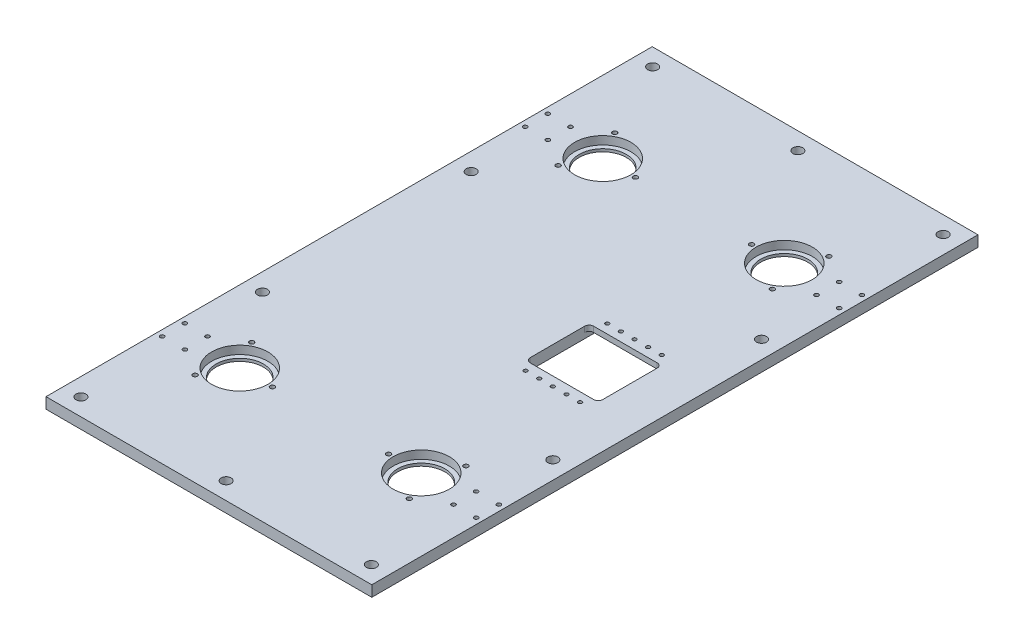
from build123d import *

# Parameters (mm, degrees)
SKETCH1_W                                          = 359
SKETCH1_H                                          = 668
BOSS_EXTRUDE1_DEPTH                                = 12
HOLE_SIZE_BASED_ON_SOCKET_HEAD_CAP_SCR_D           = 4.5
HOLE_SIZE_BASED_ON_SOCKET_HEAD_CAP_SCR_CBORE_D     = 8
HOLE_SIZE_BASED_ON_SOCKET_HEAD_CAP_SCR_CBORE_DEPTH = 4.6
SKETCH5_R                                          = 31
CUT_EXTRUDE2_DEPTH                                 = 9
SKETCH7_R                                          = 26
CUT_EXTRUDE4_DEPTH                                 = 380.368224816
M6_TAPPED_HOLE1_D                                  = 5
M6_TAPPED_HOLE1_DEPTH                              = 15
M6_TAPPED_HOLE1_TIP                                = 1.502151548
SKETCH12_R                                         = 5.5
CUT_EXTRUDE5_DEPTH                                 = 380.368224816
CUT_EXTRUDE6_DEPTH                                 = 380.368224816
CUT_EXTRUDE8_DEPTH                                 = 6
M5_TAPPED_HOLE1_D                                  = 4.2
M5_TAPPED_HOLE1_DEPTH                              = 12.4
M5_TAPPED_HOLE1_TIP                                = 1.2618073


with BuildPart() as part:
    # Sketch1 → Boss-Extrude1 (new body)
    with BuildSketch(Plane(origin=(0, 0, 0), x_dir=(1, 0, 0), z_dir=(0, 1, 0))):
        Rectangle(SKETCH1_W, SKETCH1_H)
    extrude(amount=BOSS_EXTRUDE1_DEPTH)

    # Hole size (%based on) socket head cap screw type 1 (through all)
    with Locations(Plane.XZ):
        with Locations((-173, 212.5), (-148, 212.5), (-148, 187.5), (-173, 187.5), (-173, -187.5), (-148, -187.5), (-148, -212.5), (-173, -212.5), (173, -212.5), (148, -212.5), (148, -187.5), (173, -187.5), (173, 187.5), (148, 187.5), (148, 212.5), (173, 212.5)):
            CounterBoreHole(HOLE_SIZE_BASED_ON_SOCKET_HEAD_CAP_SCR_D / 2, HOLE_SIZE_BASED_ON_SOCKET_HEAD_CAP_SCR_CBORE_D / 2, HOLE_SIZE_BASED_ON_SOCKET_HEAD_CAP_SCR_CBORE_DEPTH)

    # Sketch5 → Cut-Extrude2 (cut)
    with BuildSketch(Plane(origin=(0, 12, 0), x_dir=(1, 0, 0), z_dir=(0, 1, 0))):
        with Locations(Location((-100, -200, 0), (0, 0, 270))):
            Circle(SKETCH5_R)
        with Locations(Location((100, -200, 0), (0, 0, 90))):
            Circle(SKETCH5_R)
        with Locations(Location((100, 200, 0), (0, 0, 270))):
            Circle(SKETCH5_R)
        with Locations(Location((-100, 200, 0), (0, 0, 90))):
            Circle(SKETCH5_R)
    extrude(amount=-CUT_EXTRUDE2_DEPTH, mode=Mode.SUBTRACT)

    # Sketch7 → Cut-Extrude4 (cut, through all)
    with BuildSketch(Plane(origin=(0, 12, 0), x_dir=(1, 0, 0), z_dir=(0, 1, 0))):
        with Locations(Location((-100, 200, 0), (0, 0, 270))):
            Circle(SKETCH7_R)
        with Locations(Location((100, 200, 0), (0, 0, 270))):
            Circle(SKETCH7_R)
        with Locations(Location((100, -200, 0), (0, 0, 270))):
            Circle(SKETCH7_R)
        with Locations(Location((-100, -200, 0), (0, 0, 270))):
            Circle(SKETCH7_R)
    extrude(amount=-CUT_EXTRUDE4_DEPTH, mode=Mode.SUBTRACT)

    # M6 Tapped Hole1
    with Locations(Plane(origin=(0, 12, 0), x_dir=(1, 0, 0), z_dir=(0, 1, 0))):
        with Locations((-118, 231.176914536), (-64, 200), (-118, 168.823085464), (118, 168.823085464), (64, 200), (118, 231.176914536), (118, -231.176914536), (64, -200), (118, -168.823085464), (-118, -168.823085464), (-64, -200), (-118, -231.176914536)):
            Hole(M6_TAPPED_HOLE1_D / 2, depth=M6_TAPPED_HOLE1_DEPTH)
            with Locations((0, 0, -(M6_TAPPED_HOLE1_DEPTH + M6_TAPPED_HOLE1_TIP / 2))):  # 118° drill point
                Cone(0, M6_TAPPED_HOLE1_D / 2, M6_TAPPED_HOLE1_TIP, mode=Mode.SUBTRACT)

    # Sketch12 → Cut-Extrude5 (cut, through all)
    with BuildSketch(Plane.XZ):
        with Locations(Location((-160, 315, 0), (0, 0, 270))):
            Circle(SKETCH12_R)
        with Locations(Location((0, 315, 0), (0, 0, 270))):
            Circle(SKETCH12_R)
        with Locations(Location((-160, 115, 0), (0, 0, 270))):
            Circle(SKETCH12_R)
        with Locations(Location((-160, -115, 0), (0, 0, 270))):
            Circle(SKETCH12_R)
        with Locations(Location((-160, -315, 0), (0, 0, 270))):
            Circle(SKETCH12_R)
        with Locations(Location((0, -315, 0), (0, 0, 270))):
            Circle(SKETCH12_R)
        with Locations(Location((160, -315, 0), (0, 0, 270))):
            Circle(SKETCH12_R)
        with Locations(Location((160, -115, 0), (0, 0, 270))):
            Circle(SKETCH12_R)
        with Locations(Location((160, 115, 0), (0, 0, 270))):
            Circle(SKETCH12_R)
        with Locations(Location((160, 315, 0), (0, 0, 270))):
            Circle(SKETCH12_R)
    extrude(amount=-CUT_EXTRUDE5_DEPTH, mode=Mode.SUBTRACT)

    # Sketch13 → Cut-Extrude6 (cut, through all)
    with BuildSketch(Plane(origin=(0, 12, 0), x_dir=(1, 0, 0), z_dir=(0, 1, 0))):
        with BuildLine():
            Line((55, 35), (125, 35))
            ThreePointArc((125, 35), (128.535533906, 33.535533906), (130, 30))
            Line((130, 30), (130, -30))
            ThreePointArc((130, -30), (128.535533906, -33.535533906), (125, -35))
            Line((125, -35), (55, -35))
            ThreePointArc((55, -35), (51.464466094, -33.535533906), (50, -30))
            Line((50, -30), (50, 30))
            ThreePointArc((50, 30), (51.464466094, 33.535533906), (55, 35))
        make_face()
    extrude(amount=-CUT_EXTRUDE6_DEPTH, mode=Mode.SUBTRACT)

    # Sketch17 → Cut-Extrude8 (cut)
    with BuildSketch(Plane.XZ):
        with BuildLine():
            Line((55, -55), (125, -55))
            ThreePointArc((125, -55), (128.535533906, -53.535533906), (130, -50))
            Line((130, -50), (130, 50))
            ThreePointArc((130, 50), (128.535533906, 53.535533906), (125, 55))
            Line((125, 55), (55, 55))
            ThreePointArc((55, 55), (51.464466094, 53.535533906), (50, 50))
            Line((50, 50), (50, -50))
            ThreePointArc((50, -50), (51.464466094, -53.535533906), (55, -55))
        make_face()
    extrude(amount=-CUT_EXTRUDE8_DEPTH, mode=Mode.SUBTRACT)

    # M5 Tapped Hole1
    with Locations(Plane(origin=(0, 6, 0), x_dir=(-1, 0, 0), z_dir=(0, -1, 0))):
        with Locations((-120, 45), (-105, 45), (-90, 45), (-75, 45), (-60, 45), (-60, -45), (-75, -45), (-90, -45), (-105, -45), (-120, -45)):
            Hole(M5_TAPPED_HOLE1_D / 2, depth=M5_TAPPED_HOLE1_DEPTH)
            with Locations((0, 0, -(M5_TAPPED_HOLE1_DEPTH + M5_TAPPED_HOLE1_TIP / 2))):  # 118° drill point
                Cone(0, M5_TAPPED_HOLE1_D / 2, M5_TAPPED_HOLE1_TIP, mode=Mode.SUBTRACT)


solid = part.part
